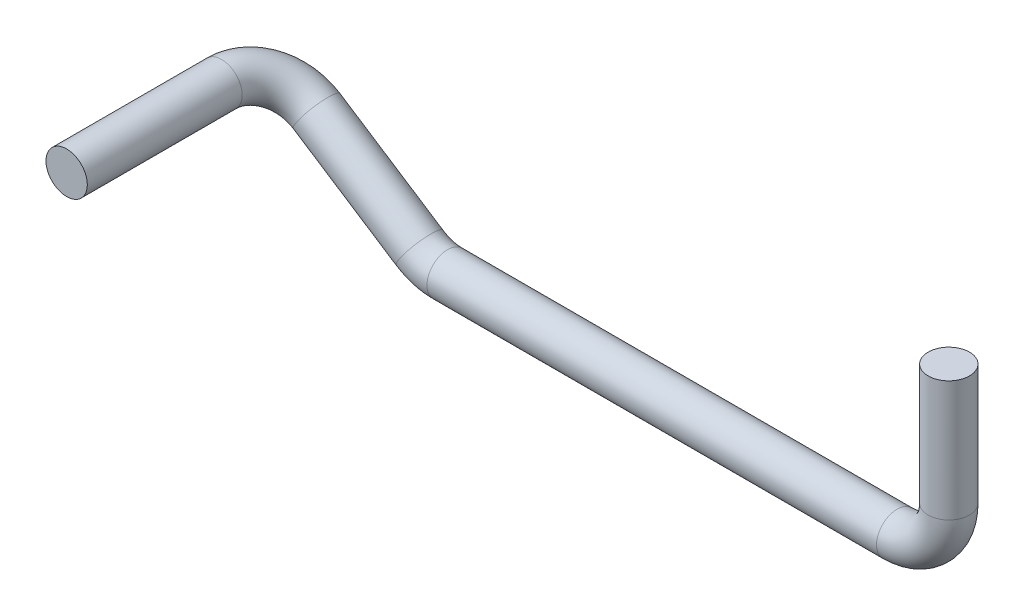
from build123d import *

# Parameters (mm, degrees)
SWEEP_1_PROFILE_R = 6


with BuildPart() as part:
    # 扫描1: sweep along a curve in space
    with BuildLine() as sweep_1_path:
        Line((150, 15, 0), (150, 50, 0))
        ThreePointArc((135, 0, 0), (145.606601718, 4.393398282, 0), (150, 15, 0))
        Line((4.442940339, 0, 0), (135, 0, 0))
        ThreePointArc((4.442940339, 0, 0), (0.182941192, 0.617635547, 0), (-3.726241034, 2.41967903, 0))
        Line((-3.726241034, 2.41967903, 0), (-33.618877196, 21.830818627, 0))
        ThreePointArc((-33.618877196, 21.830818627, 0), (-42.514507463, 27.607302173, 4.393398282), (-46.199198166, 30, 15))
        Line((-46.199198166, 30, 15), (-46.199198166, 30, 60))
    # 扫描1 profile (on start of the path) → 扫描1 (sweep)
    with BuildSketch(Plane(origin=(-46.199198166, 30, 60), x_dir=(0, -1, 0), z_dir=(0, 0, -1))):
        Circle(SWEEP_1_PROFILE_R)
    sweep(path=sweep_1_path.line)


solid = part.part
